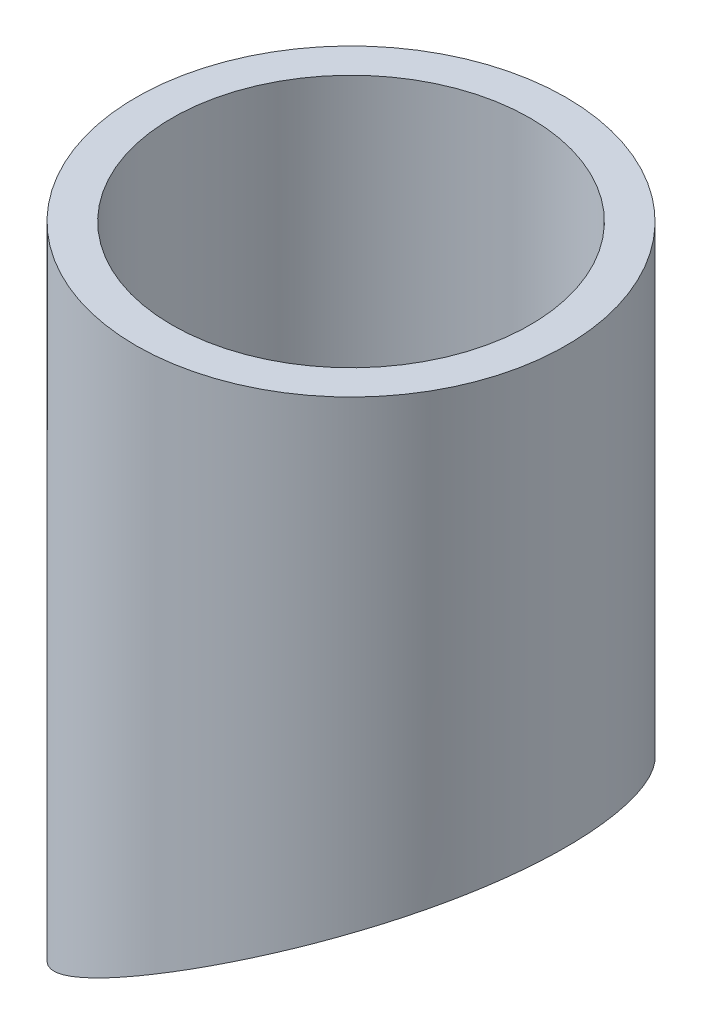
SolidWorks part; units mm, degrees
material "不锈钢管60×5"
ref_plane "Front Plane" through (0, 0, 0) normal (0, 0, 1) x (1, 0, 0)
ref_plane "Top Plane" through (0, 0, 0) normal (0, 1, 0) x (1, 0, 0)
ref_plane "Right Plane" through (0, 0, 0) normal (1, 0, 0) x (0, 0, -1)
sketch "Sketch2" plane through (0, 0, 0) normal (0, 1, 0) x (1, 0, 0)
  circle A0 centre (0, 0) radius 25
  circle A1 centre (0, 0) radius 30
  dimension "D1" = 50
  dimension "D2" = 60
extrude "Boss-Extrude1" add sketch "Sketch2" along normal blind 300
cosmetic thread "Cosmetic Thread1" parameters "D1"=25, "D2"=56.656
sketch "Sketch3" plane through (0, 0, 0) normal (0, 0, 1) x (1, 0, 0)
  line L1 (0, 399.5609) -> (0, 223.8187) construction
  line L3 (0, 223.8187) -> (189.75, -104.8379) construction
  circle A3 centre (189.75, -104.8379) radius 379.5
  dimension "D1" = 150
  dimension "D2" = 379.5
extrude "Cut-Extrude1" cut sketch "Sketch3" against normal through all both and the other way through all
